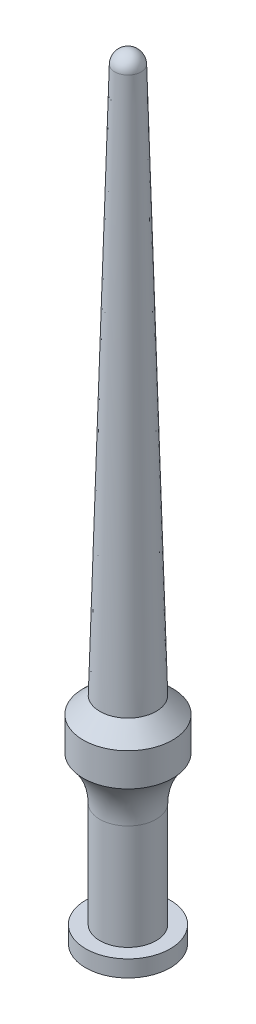
SolidWorks part; units mm, degrees
material "Q235B"
ref_plane "Front Plane" through (0, 0, 0) normal (0, 0, 1) x (1, 0, 0)
ref_plane "Top Plane" through (0, 0, 0) normal (0, 1, 0) x (1, 0, 0)
ref_plane "Right Plane" through (0, 0, 0) normal (1, 0, 0) x (0, 0, -1)
sketch "Sketch1" plane through (0, 0, 0) normal (0, 0, 1) x (1, 0, 0)
  line L0 (0, 0) -> (25.5, 0)
  line L1 (25.5, 0) -> (25.5, 10)
  line L2 (25.5, 10) -> (17, 10)
  line L3 (17, 10) -> (17, 73.5425)
  line L4 (27, 100) -> (27, 120)
  line L5 (27, 120) -> (17, 130)
  line L6 (17, 130) -> (7.997, 460.218)
  line L7 (0, 468) -> (0, 0)
  line L8 (0, 0) -> (0, -16.2031) construction
  arc A0 (17, 73.5425) -> (27, 100) centre (57, 73.5425) cw
  arc A1 (7.997, 460.218) -> (0, 468) centre (0, 460) ccw
  dimension "D1" = 51
  dimension "D5" = 8
  dimension "D11" = 40
  dimension "D2" = 34
  dimension "D3" = 54
  dimension "D4" = 34
  dimension "D6" = 10
  dimension "D7" = 90
  dimension "D8" = 20
  dimension "D9" = 468
  dimension "D10" = 45
revolve "Revolve1" add sketch "Sketch1" angle 360 about L8
